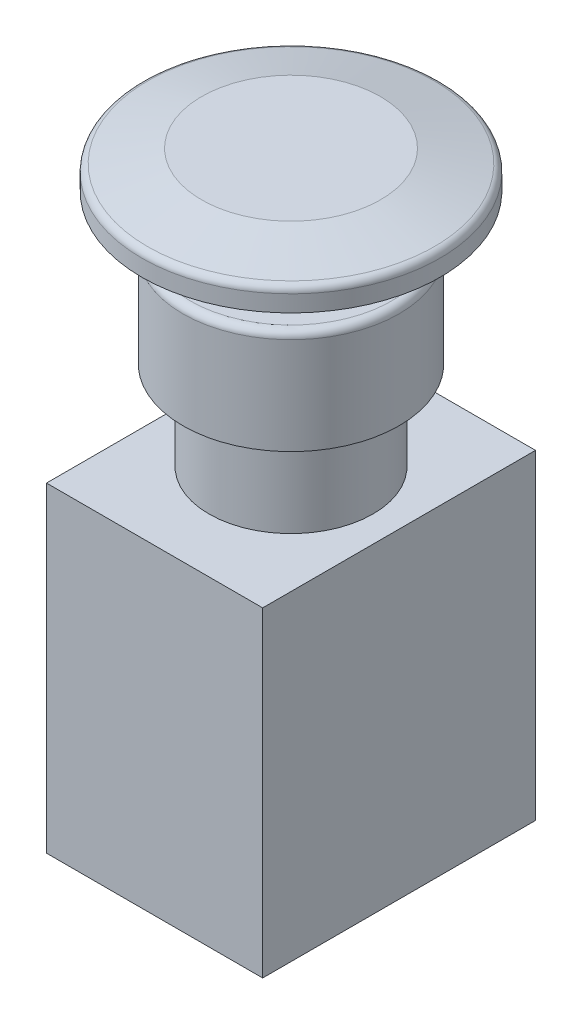
from build123d import *

# Parameters (mm, degrees)
SKETCH1_R           = 14.5
BOSS_EXTRUDE1_DEPTH = 14
SKETCH2_R           = 11
BOSS_EXTRUDE2_DEPTH = 6
SKETCH3_R           = 20
BOSS_EXTRUDE3_DEPTH = 5
FILLET1_R           = 1
BOSS_EXTRUDE4_START = 12
SKETCH5_R           = 11
BOSS_EXTRUDE4_DEPTH = 12
SKETCH6_W           = 29
SKETCH6_H           = 36.6
BOSS_EXTRUDE5_DEPTH = 43


with BuildPart() as part:
    # Sketch1 → Boss-Extrude1 (new body)
    with BuildSketch(Plane(origin=(0, 0, 0), x_dir=(1, 0, 0), z_dir=(0, 1, 0))):
        with Locations(Location((0, 0, 0), (0, 0, 270))):
            Circle(SKETCH1_R)
    extrude(amount=BOSS_EXTRUDE1_DEPTH)

    # Sketch2 → Boss-Extrude2 (add)
    with BuildSketch(Plane(origin=(0, 14, 0), x_dir=(1, 0, 0), z_dir=(0, 1, 0))):
        with Locations(Location((0, 0, 0), (0, 0, 270))):
            Circle(SKETCH2_R)
    extrude(amount=BOSS_EXTRUDE2_DEPTH)

    # Sketch3 → Boss-Extrude3 (add)
    with BuildSketch(Plane(origin=(0, 20, 0), x_dir=(1, 0, 0), z_dir=(0, 1, 0))):
        with Locations(Location((0, 0, 0), (0, 0, 270))):
            Circle(SKETCH3_R)
    extrude(amount=BOSS_EXTRUDE3_DEPTH)

    # Sketch4 → Cut-Revolve1 (revolve, cut)
    with BuildSketch(Plane.XY, mode=Mode.PRIVATE) as cut_revolve1_sk:
        Polygon((-12, 25), (-20, 25), (-20, 23), align=None)
    revolve(cut_revolve1_sk.sketch.rotate(Axis((0, 0, 0), (0, 1, 0)), 270), axis=Axis((0, 0, 0), (0, 1, 0)), mode=Mode.SUBTRACT)

    # Fillet1
    fillet1_edges = [part.edges().sort_by_distance(p)[0] for p in [
        (-20, 23, 0),
        (0, 14, -14.5),
    ]]
    fillet(fillet1_edges, radius=FILLET1_R)

    # Sketch5 → Boss-Extrude4 (add)
    with BuildSketch(Plane.XZ.offset(BOSS_EXTRUDE4_START)):
        with Locations(Location((0, 0, 0), (0, 0, 90))):
            Circle(SKETCH5_R)
    extrude(amount=-BOSS_EXTRUDE4_DEPTH)

    # Sketch6 → Boss-Extrude5 (add)
    with BuildSketch(Plane.XZ.offset(12)):
        Rectangle(SKETCH6_W, SKETCH6_H)
    extrude(amount=BOSS_EXTRUDE5_DEPTH)


solid = part.part
